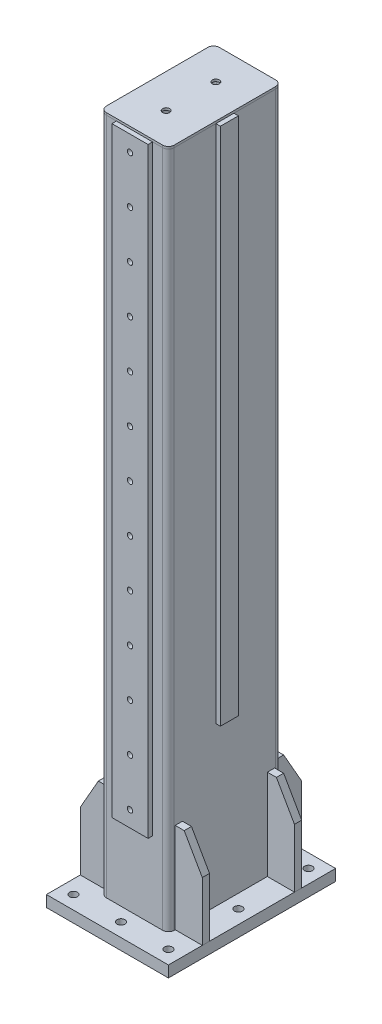
SolidWorks part; units mm, degrees
material "Q235-B"
ref_plane "前视基准面" through (0, 0, 0) normal (0, 0, 1) x (1, 0, 0)
ref_plane "上视基准面" through (0, 0, 0) normal (0, 1, 0) x (1, 0, 0)
ref_plane "右视基准面" through (0, 0, 0) normal (1, 0, 0) x (0, 0, -1)
other "Configuration Table"
sketch "草图1" plane through (0, 0, 0) normal (0, 0, 1) x (1, 0, 0)
  line L0 (0, 0) -> (0, 1500)
  dimension "D1" = 1500
other "Rhs RHS250X150X6.3(1)"
ref_plane "基准面1" through (0, 0, 0) normal (0, 1, 0) x (-1, 0, 0)
sketch "Sketch140" plane through (0, 0, 0) normal (0, 1, 0) x (-1, 0, 0)
  line L0 (-62.4, -118.7) -> (62.4, -118.7)
  line L1 (-68.7, -112.4) -> (-68.7, 112.4)
  line L2 (62.4, 118.7) -> (-62.4, 118.7)
  line L3 (68.7, 112.4) -> (68.7, -112.4)
  line L4 (-62.4, -125) -> (62.4, -125)
  line L5 (-75, -112.4) -> (-75, 112.4)
  line L6 (62.4, 125) -> (-62.4, 125)
  line L7 (75, 112.4) -> (75, -112.4)
  line L8 (-75, 0) -> (-68.7, 0) construction
  line L9 (-68.7, 0) -> (68.7, 0) construction
  line L10 (68.7, 0) -> (75, 0) construction
  line L11 (0, 125) -> (0, 118.7) construction
  line L12 (0, 118.7) -> (0, -118.7) construction
  line L13 (0, -118.7) -> (0, -125) construction
  arc A0 (75, 112.4) -> (62.4, 125) centre (62.4, 112.4) ccw
  arc A1 (62.4, -125) -> (75, -112.4) centre (62.4, -112.4) ccw
  arc A2 (-75, -112.4) -> (-62.4, -125) centre (-62.4, -112.4) ccw
  arc A3 (-62.4, 125) -> (-75, 112.4) centre (-62.4, 112.4) ccw
  arc A4 (-62.4, 118.7) -> (-68.7, 112.4) centre (-62.4, 112.4) ccw
  arc A5 (68.7, 112.4) -> (62.4, 118.7) centre (62.4, 112.4) ccw
  arc A6 (62.4, -118.7) -> (68.7, -112.4) centre (62.4, -112.4) ccw
  arc A7 (-68.7, -112.4) -> (-62.4, -118.7) centre (-62.4, -112.4) ccw
  point P6 (75, -125)
  point P33 (-75, -125)
  point P35 (-75, 125)
  point P36 (75, 125)
  point P37 (0, 0)
  point P38 (0, 0)
  dimension "D1" = 12.6
  dimension "Thickness" = 6.3
  dimension "V_leg" = 250
  dimension "H_leg" = 150
sketch "草图50" plane through (0, 0, 0) normal (0, -1, 0) x (1, 0, 0)
  line L0 (-62.4, 125) -> (62.4, 125) construction
  line L1 (-135, -185) -> (135, -185)
  line L2 (-135, -185) -> (-135, 185)
  line L3 (-135, 185) -> (135, 185)
  line L4 (135, -185) -> (135, 185)
  line L5 (0, 185) -> (0, -185) construction
  line L6 (-135, 0) -> (135, 0) construction
  line L7 (75, 112.4) -> (75, -112.4) construction
  point P0 (0, 0)
  dimension "D1" = 60
  dimension "D2" = 60
extrude "凸台-拉伸1" add sketch "草图50" along normal blind 25 separate body
sketch "草图51" plane through (50, 0, 125) normal (0, 0, 1) x (1, 0, 0)
  line L1 (-90, 1500) -> (-10, 1500)
  line L2 (-90, 1500) -> (-90, 170)
  line L3 (-90, 170) -> (-10, 170)
  line L4 (-10, 1500) -> (-10, 170)
  line L6 (-125, 1500) -> (-125, 0) construction
  line L7 (-112.4, 1500) -> (12.4, 1500) construction
  dimension "D1" = 80
  dimension "D2" = 35
  dimension "D3" = 1330
extrude "凸台-拉伸2" add sketch "草图51" along normal blind 10 separate body
ref_plane "基准面2" through (0, 0, 110) normal (0, 0, 1) x (1, 0, 0)
sketch "草图52" plane through (0, 0, 110) normal (0, 0, 1) x (1, 0, 0)
  line L0 (75, 200) -> (95, 200)
  line L1 (75, 1500) -> (75, 0) construction
  line L2 (95, 200) -> (135, 130)
  line L3 (135, 130) -> (135, 0)
  line L4 (135, 0) -> (75, 0)
  line L5 (135, 0) -> (-135, 0) construction
  line L6 (75, 0) -> (75, 200)
  line L7 (0, 0) -> (0, -25) construction
  line L8 (135, -25) -> (-135, -25) construction
  line L9 (-75, 0) -> (-75, 200)
  line L10 (-135, 0) -> (-75, 0)
  line L11 (-135, 130) -> (-135, 0)
  line L12 (-95, 200) -> (-135, 130)
  line L13 (-75, 200) -> (-95, 200)
  dimension "D1" = 20
  dimension "D2" = 130
  dimension "D3" = 200
extrude "凸台-拉伸3" add sketch "草图52" against normal blind 16 separate body
ref_plane "基准面3" through (60, 0, 0) normal (1, 0, 0) x (0, 0, -1)
mirror "镜向2" about plane through (0, 0, 0) normal (0, 0, 1) of bodies 109 110
sketch "草图56" plane through (0, -25, 0) normal (0, -1, 0) x (-1, 0, 0)
  line L0 (135, 185) -> (-135, 185) construction
  line L1 (-135, 185) -> (-135, -185) construction
  line L2 (-105, 155) -> (0, 155) construction
  line L3 (-105, 155) -> (-105, 0) construction
  point P0 (-105, 155)
  point P12 (0, 155)
  point P13 (105, 155)
  point P15 (105, 0)
  point P16 (0, -155)
  point P17 (105, -155)
  point P18 (-105, 0)
  point P19 (-105, -155)
  point P25 (0, 0) [skipped]
  dimension "D1" = 30
  dimension "D2" = 30
  dimension "D5" = 105
  dimension "D6" = 155
  dimension "D7" = 30
  dimension "D3" = 3
  dimension "D4" = 3
hole_wizard "M20 螺纹孔1" positions "草图56" profile "草图55" tap size "M20" standard "GB"
cosmetic thread "孔螺纹线1"
cosmetic thread "孔螺纹线2"
cosmetic thread "孔螺纹线3"
cosmetic thread "孔螺纹线4"
cosmetic thread "孔螺纹线5"
cosmetic thread "孔螺纹线6"
cosmetic thread "孔螺纹线7"
cosmetic thread "孔螺纹线8"
sketch "草图55" plane through (105, -25, -155) normal (1, 0, 0) x (0, 0, -1)
  line L0 (0, 0) -> (0, 25.001)
  line L1 (0, 25.001) -> (8.75, 25.001)
  line L2 (8.75, 25.001) -> (8.75, 0)
  line L5 (8.75, 0) -> (0, 0)
  line L11 (0, -6.35) -> (0, 107.95) construction
  dimension "通孔螺纹孔钻头直径" = 17.5
  dimension "通孔螺纹孔钻头深度" = 25.001
sketch "草图57" plane through (75, 0, 0) normal (1, 0, 0) x (0, 0, -1)
  line L0 (-112.4, 1500) -> (112.4, 1500) construction
  line L1 (-20, 1500) -> (20, 1500)
  line L2 (-20, 1500) -> (-20, 350)
  line L3 (-20, 350) -> (20, 350)
  line L4 (20, 1500) -> (20, 350)
  line L5 (-125, 1500) -> (-125, 0) construction
  dimension "D1" = 40
  dimension "D2" = 105
  dimension "D3" = 1150
extrude "凸台-拉伸5" add sketch "草图57" along normal blind 10 separate body
sketch "草图58" plane through (60, 0, 0) normal (1, 0, 0) x (0, 0, -1)
  line L0 (125, 200) -> (145, 200)
  line L1 (125, 1500) -> (125, 0) construction
  line L2 (145, 200) -> (185, 130)
  line L3 (185, 130) -> (185, 0)
  line L4 (185, 0) -> (125, 0)
  line L5 (125, 0) -> (125, 200)
  dimension "D1" = 20
  dimension "D2" = 130
  dimension "D3" = 200
extrude "凸台-拉伸6" add sketch "草图58" against normal blind 16 separate body
mirror "镜向3" about plane through (0, 0, 0) normal (1, 0, 0) of bodies 117
sketch "草图59" plane through (0, 0, -125) normal (0, 0, -1) x (-1, 0, 0)
  line L0 (-75, 350) -> (-75, 1500) construction
  line L1 (-35, 950) -> (35, 950) construction
  line L2 (-35, 950) -> (-35, 810) construction
  line L3 (-35, 810) -> (35, 810) construction
  line L4 (35, 950) -> (35, 810) construction
  line L5 (-62.4, 1500) -> (62.4, 1500) construction
  line L6 (-35, 950) -> (35, 950) construction
  line L7 (-35, 950) -> (-35, 810) construction
  line L8 (0, 950) -> (0, 810) construction
  circle A0 centre (-35, 950) radius 8.75
  circle A1 centre (35, 950) radius 8.75
  circle A2 centre (35, 810) radius 8.75
  circle A3 centre (-35, 810) radius 8.75
  dimension "D5" = 17.5
  dimension "D10" = 35
  dimension "D1" = 140
  dimension "D2" = 70
  dimension "D3" = 40
  dimension "D4" = 550
  dimension "D8" = 70
  dimension "D9" = 140
  dimension "D6" = 2
  dimension "D7" = 2
extrude "切除-拉伸1" cut sketch "草图59" against normal up to next (6.3 mm away)
sketch "草图60" plane through (-75, 0, 0) normal (-1, 0, 0) x (0, 0, 1)
  line L0 (-125, 1500) -> (-125, 0) construction
  circle A0 centre (-65, 940) radius 17.5
  circle A1 centre (-65, 820) radius 17.5
  dimension "D3" = 35
  dimension "D4" = 35
  dimension "D1" = 120
  dimension "D2" = 60
  dimension "D5" = 560
  dimension "D6" = 60
extrude "切除-拉伸2" cut sketch "草图60" against normal up to next (6.3 mm away)
sketch "草图63" plane through (0, 0, 135) normal (0, 0, 1) x (1, 0, 0)
  line L0 (40, 1500) -> (-40, 1500) construction
  line L1 (40, 170) -> (40, 1500) construction
  line L2 (0, 1465) -> (0, 1360) construction
  point P0 (0, 1465)
  point P13 (0, 1360)
  point P14 (0, 1255)
  point P15 (0, 1150)
  point P16 (0, 1045)
  point P17 (0, 940)
  point P18 (0, 835)
  point P19 (0, 730)
  point P20 (0, 625)
  point P21 (0, 520)
  point P22 (0, 415)
  point P23 (0, 310)
  point P24 (0, 205)
  dimension "D1" = 35
  dimension "D2" = 40
  dimension "D4" = 105
  dimension "D3" = 13
hole_wizard "M14 螺纹孔1" positions "草图63" profile "草图62" tap size "M14" standard "GB" end condition up to next
sketch "草图62" plane through (0, 1465, 135) normal (1, 0, 0) x (0, -1, 0)
  line L0 (0, 0) -> (0, 10)
  line L1 (0, 10) -> (6, 10)
  line L2 (6, 10) -> (6, 0)
  line L5 (6, 0) -> (0, 0)
  line L11 (0, -6.35) -> (0, 107.95) construction
  dimension "通孔螺纹孔钻头直径" = 12
  dimension "通孔螺纹孔钻头深度" = 10
cosmetic thread "孔螺纹线9"
cosmetic thread "孔螺纹线10"
cosmetic thread "孔螺纹线11"
cosmetic thread "孔螺纹线12"
cosmetic thread "孔螺纹线13"
cosmetic thread "孔螺纹线14"
cosmetic thread "孔螺纹线15"
cosmetic thread "孔螺纹线16"
cosmetic thread "孔螺纹线17"
cosmetic thread "孔螺纹线18"
cosmetic thread "孔螺纹线19"
cosmetic thread "孔螺纹线20"
cosmetic thread "孔螺纹线21"
sketch "草图64" plane through (0, 1500, 0) normal (0, 1, 0) x (1, 0, 0)
  line L4 (-62.4, -125) -> (62.4, -125)
  line L5 (75, -112.4) -> (75, 112.4)
  line L6 (62.4, 125) -> (-62.4, 125)
  line L7 (-75, 112.4) -> (-75, -112.4)
  line L8 (-62.4, -125) -> (62.4, -125)
  line L9 (75, -112.4) -> (75, 112.4)
  line L10 (62.4, 125) -> (-62.4, 125)
  line L11 (-75, 112.4) -> (-75, -112.4)
  arc A4 (-75, -112.4) -> (-62.4, -125) centre (-62.4, -112.4) ccw
  arc A5 (62.4, -125) -> (75, -112.4) centre (62.4, -112.4) ccw
  arc A6 (75, 112.4) -> (62.4, 125) centre (62.4, 112.4) ccw
  arc A7 (-62.4, 125) -> (-75, 112.4) centre (-62.4, 112.4) ccw
  arc A8 (-75, -112.4) -> (-62.4, -125) centre (-62.4, -112.4) ccw
  arc A9 (62.4, -125) -> (75, -112.4) centre (62.4, -112.4) ccw
  arc A10 (75, 112.4) -> (62.4, 125) centre (62.4, 112.4) ccw
  arc A11 (-62.4, 125) -> (-75, 112.4) centre (-62.4, 112.4) ccw
  dimension "D1" = 0
extrude "凸台-拉伸7" add sketch "草图64" along normal blind 5 separate body
sketch "草图67" plane through (0, 1505, 0) normal (0, 1, 0) x (1, 0, 0)
  line L0 (-75, 112.4) -> (-75, -112.4) construction
  point P0 (0, 55)
  point P2 (0, -55)
  dimension "D1" = 75
  dimension "D2" = 75
  dimension "D3" = 55
  dimension "D4" = 55
hole_wizard "M18 螺纹孔1" positions "草图67" profile "草图66" tap size "M18" standard "GB"
sketch "草图66" plane through (0, 1505, -55) normal (1, 0, 0) x (0, 0, 1)
  line L0 (0, 0) -> (0, 53.1567)
  line L1 (0, 53.1567) -> (7.75, 48.5)
  line L2 (7.75, 48.5) -> (7.75, 0)
  line L5 (7.75, 0) -> (0, 0)
  line L10 (0, 53.1567) -> (-7.75, 48.5) construction
  line L11 (0, -6.35) -> (0, 107.95) construction
  dimension "螺纹孔钻头直径" = 15.5
  dimension "螺纹孔钻头深度" = 48.5
  dimension "导头角度" = 118
cosmetic thread "孔螺纹线22"
cosmetic thread "孔螺纹线23"
